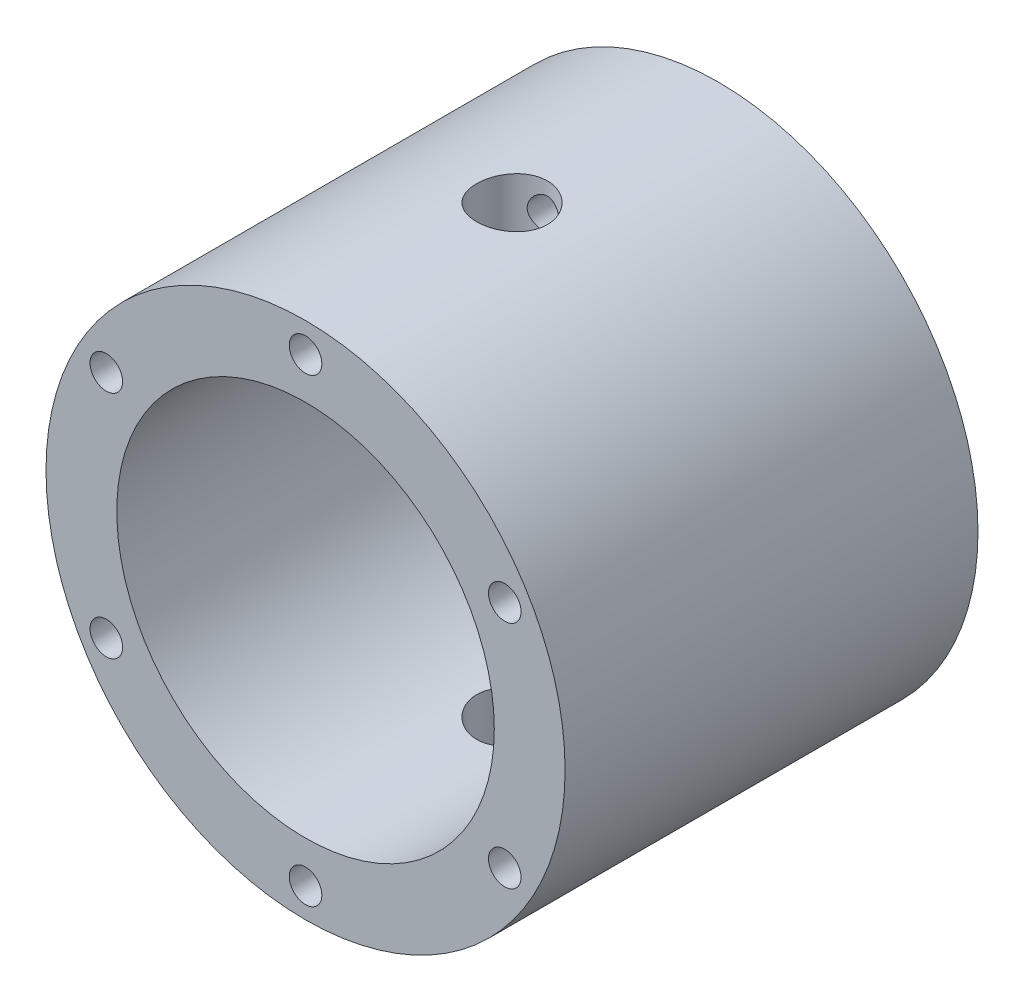
SolidWorks part; units mm, degrees
ref_plane "Front Plane" through (0, 0, 0) normal (0, 0, 1) x (1, 0, 0)
ref_plane "Top Plane" through (0, 0, 0) normal (0, 1, 0) x (1, 0, 0)
ref_plane "Right Plane" through (0, 0, 0) normal (1, 0, 0) x (0, 0, -1)
sketch "Sketch1" plane through (0, 0, 0) normal (0, 0, 1) x (1, 0, 0)
  circle A0 centre (0, 0) radius 110
  circle A1 centre (0, 0) radius 80
  circle A2 centre (0, 0) radius 97.5 construction
  circle A3 centre (0, 97.5) radius 6.9
  circle A4 centre (84.4375, 48.75) radius 6.9
  circle A5 centre (84.4375, -48.75) radius 6.9
  circle A6 centre (0, -97.5) radius 6.9
  circle A7 centre (-84.4375, -48.75) radius 6.9
  circle A8 centre (-84.4375, 48.75) radius 6.9
  point P20 (0, 0)
  dimension "D1" = 220
  dimension "D2" = 160
  dimension "D3" = 195
  dimension "D4" = 13.8
extrude "Boss-Extrude1" add sketch "Sketch1" along normal blind 175
sketch "Sketch2" plane through (0, 0, 0) normal (0, 1, 0) x (1, 0, 0)
  line L1 (110, 0) -> (-110, 0) construction
  circle A0 centre (0, -87.5) radius 15
  dimension "D1" = 30
  dimension "D2" = 87.5
extrude "Cut-Extrude1" cut sketch "Sketch2" against normal mid plane 2000
